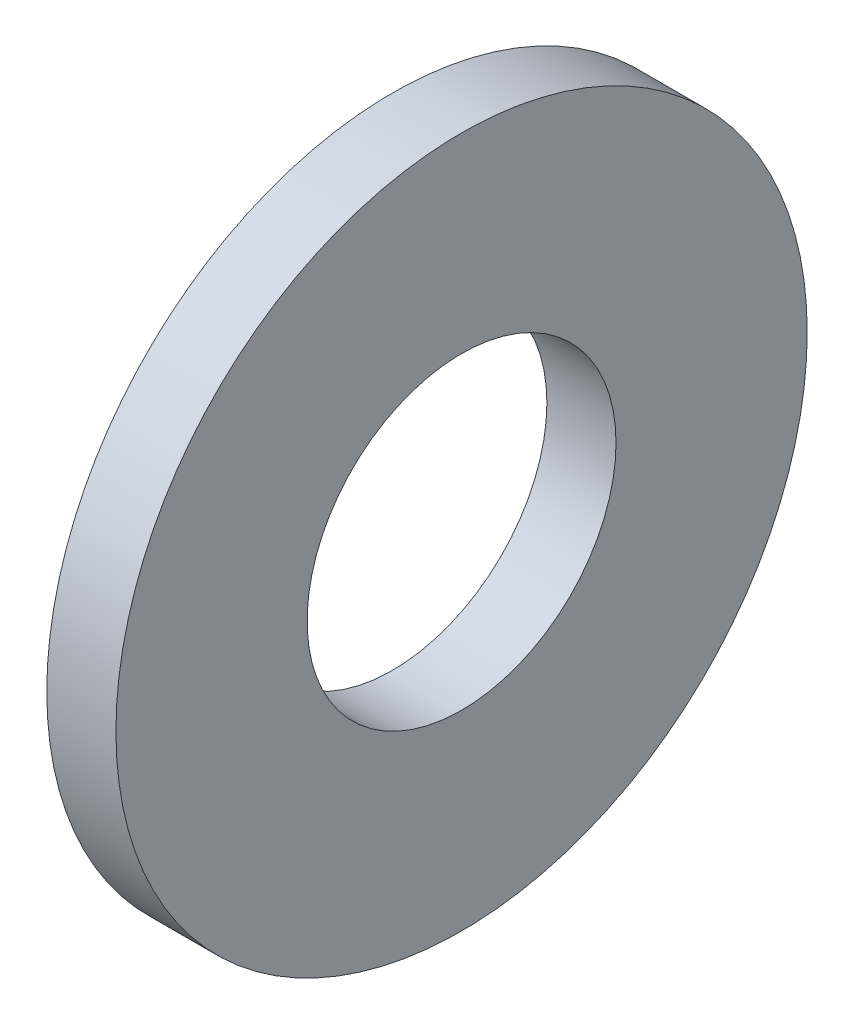
from build123d import *

# Parameters (mm, degrees)
SKETCH1_R          = 8
SKETCH1_R_2        = 3.575
BASE_EXTRUDE_DEPTH = 1.6


with BuildPart() as part:
    # Sketch1 → Base-Extrude (new body)
    with BuildSketch(Plane(origin=(0, 0, 0), x_dir=(0, 0, -1), z_dir=(1, 0, 0))):
        Circle(SKETCH1_R)
        Circle(SKETCH1_R_2, mode=Mode.SUBTRACT)
    extrude(amount=BASE_EXTRUDE_DEPTH)


solid = part.part
